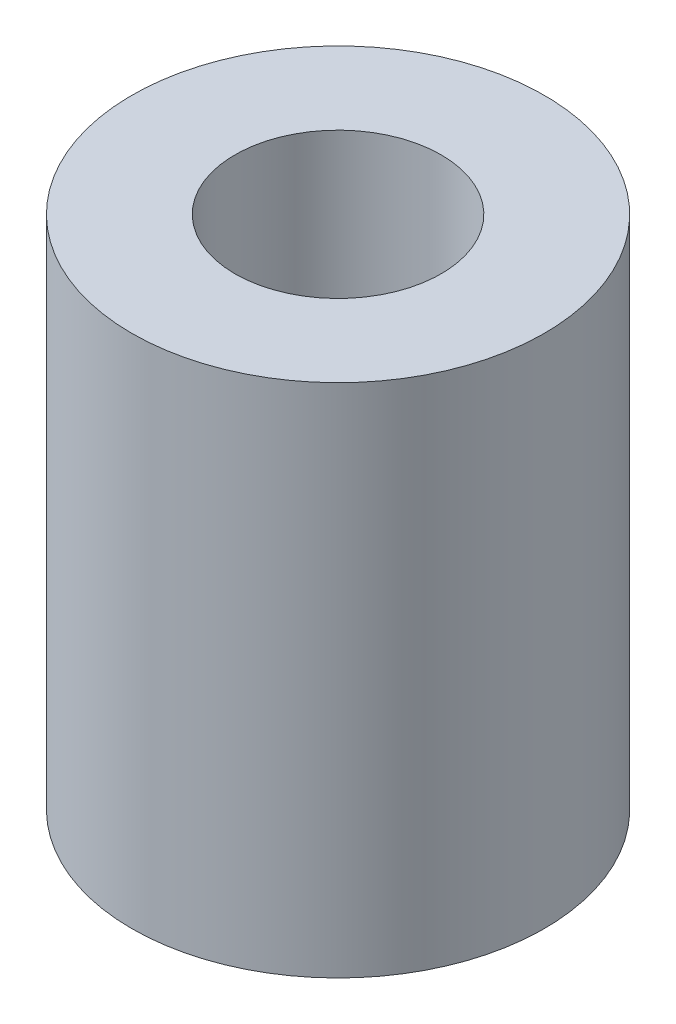
from build123d import *

# Parameters (mm, degrees)
SKETCH1_R           = 20
SKETCH1_R_2         = 10
BOSS_EXTRUDE1_DEPTH = 50


with BuildPart() as part:
    # Sketch1 → Boss-Extrude1 (new body)
    with BuildSketch(Plane(origin=(0, 0, 0), x_dir=(1, 0, 0), z_dir=(0, 1, 0))):
        with Locations(Location((0, 0, 0), (0, 0, 270))):
            Circle(SKETCH1_R)
        with Locations(Location((0, 0, 0), (0, 0, 270))):
            Circle(SKETCH1_R_2, mode=Mode.SUBTRACT)
    extrude(amount=BOSS_EXTRUDE1_DEPTH)


solid = part.part
